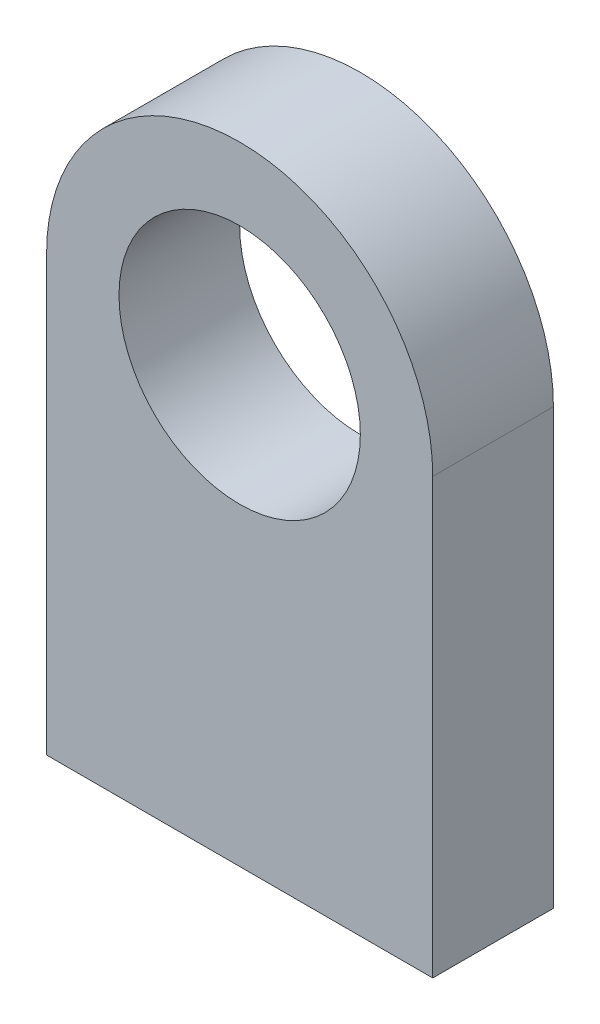
from build123d import *

# Parameters (mm, degrees)
SKETCH_1_R      = 5
EXTRUDE_1_DEPTH = 2.5


with BuildPart() as part:
    # 草图1 → 凸台-拉伸1 (new, symmetric)
    with BuildSketch(Plane.XY):
        with BuildLine():
            Line((8, 0), (8, 18))
            ThreePointArc((8, 18), (0, 26), (-8, 18))
            Line((-8, 18), (-8, 0))
            Line((-8, 0), (8, 0))
        make_face()
        with Locations((0, 18)):
            Circle(SKETCH_1_R, mode=Mode.SUBTRACT)
    extrude(amount=EXTRUDE_1_DEPTH, both=True)


solid = part.part
